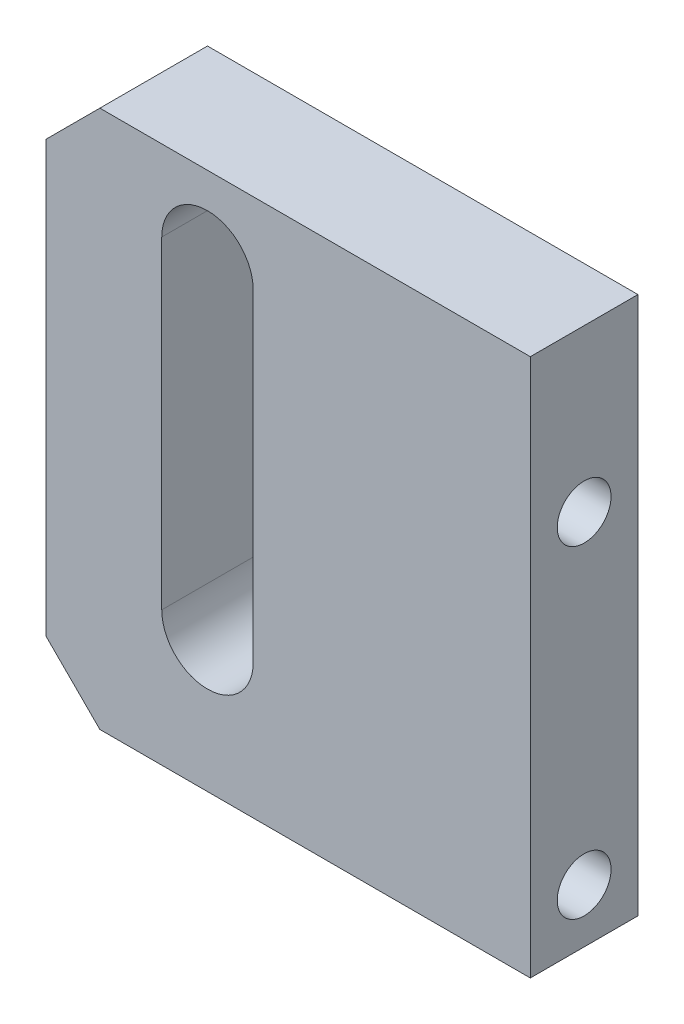
from build123d import *

# Parameters (mm, degrees)
SKETCH1_W             = 45
SKETCH1_H             = 50
BOSS_EXTRUDE1_DEPTH   = 10
CUT_EXTRUDE1_DEPTH    = 59.854546763
CHAMFER1_SIZE         = 5
M6_TAPPED_HOLE1_D     = 5
M6_TAPPED_HOLE1_DEPTH = 19
M6_TAPPED_HOLE1_TIP   = 1.502151548


with BuildPart() as part:
    # Sketch1 → Boss-Extrude1 (new body)
    with BuildSketch(Plane.XY):
        with Locations((-10.287049861, 22.842105263)):
            Rectangle(SKETCH1_W, SKETCH1_H)
    extrude(amount=BOSS_EXTRUDE1_DEPTH)

    # Sketch2 → Cut-Extrude1 (cut, through all)
    with BuildSketch(Plane.XY.offset(10)):
        with BuildLine():
            Line((-13.537049861, 40.342105263), (-13.537049861, 10.342105263))
            ThreePointArc((-13.537049861, 10.342105263), (-17.787049861, 6.092105263), (-22.037049861, 10.342105263))
            Line((-22.037049861, 10.342105263), (-22.037049861, 40.342105263))
            ThreePointArc((-22.037049861, 40.342105263), (-17.787049861, 44.592105263), (-13.537049861, 40.342105263))
        make_face()
    extrude(amount=-CUT_EXTRUDE1_DEPTH, mode=Mode.SUBTRACT)

    # Chamfer1
    chamfer1_edges = [part.edges().sort_by_distance(p)[0] for p in [
        (-32.787049861, 47.842105263, 5),
        (-32.787049861, -2.157894737, 5),
    ]]
    chamfer(chamfer1_edges, length=CHAMFER1_SIZE)

    # M6 Tapped Hole1
    with Locations(Plane(origin=(12.212950139, 0, 0), x_dir=(0, 0, -1), z_dir=(1, 0, 0))):
        with Locations((-5, 32.842105263), (-5, 2.842105263)):
            Hole(M6_TAPPED_HOLE1_D / 2, depth=M6_TAPPED_HOLE1_DEPTH)
            with Locations((0, 0, -(M6_TAPPED_HOLE1_DEPTH + M6_TAPPED_HOLE1_TIP / 2))):  # 118° drill point
                Cone(0, M6_TAPPED_HOLE1_D / 2, M6_TAPPED_HOLE1_TIP, mode=Mode.SUBTRACT)


solid = part.part
